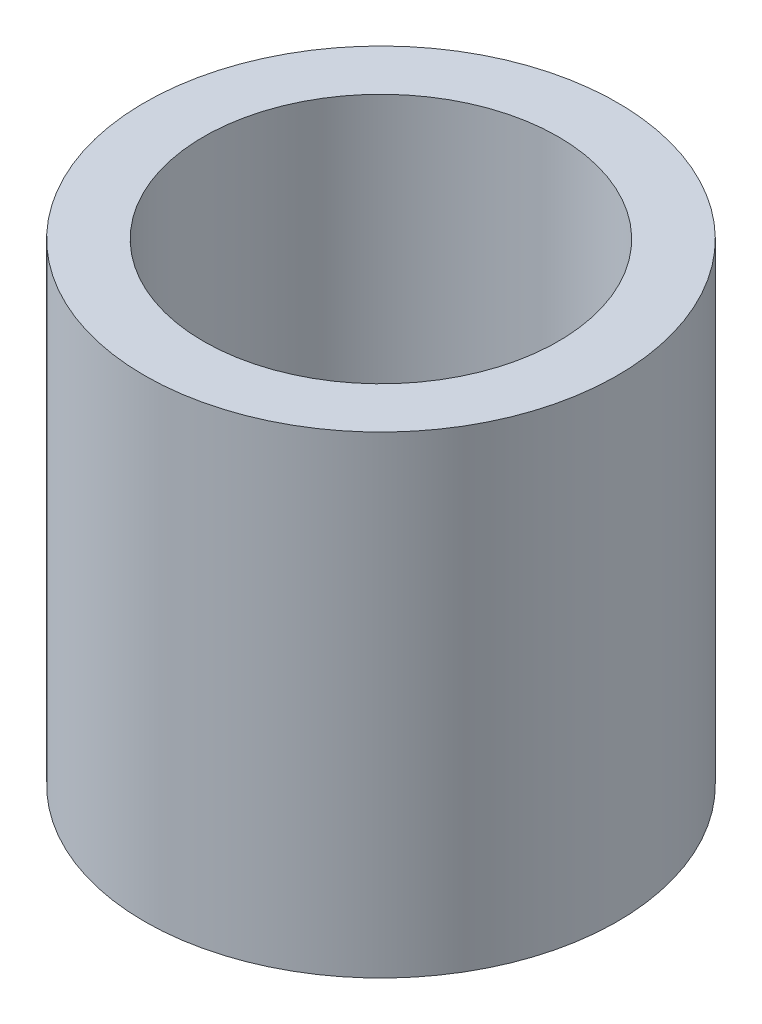
SolidWorks part; units mm, degrees
material "普通碳钢"
ref_plane "前视基准面" through (0, 0, 0) normal (0, 0, 1) x (1, 0, 0)
ref_plane "上视基准面" through (0, 0, 0) normal (0, 1, 0) x (1, 0, 0)
ref_plane "右视基准面" through (0, 0, 0) normal (1, 0, 0) x (0, 0, -1)
other "Configuration Table"
sketch "草图1" plane through (0, 0, 0) normal (0, 1, 0) x (1, 0, 0)
  circle A0 centre (0, 0) radius 3
  circle A1 centre (0, 0) radius 4
  dimension "D1" = 6
  dimension "D2" = 8
extrude "凸台-拉伸1" add sketch "草图1" along normal blind 8
